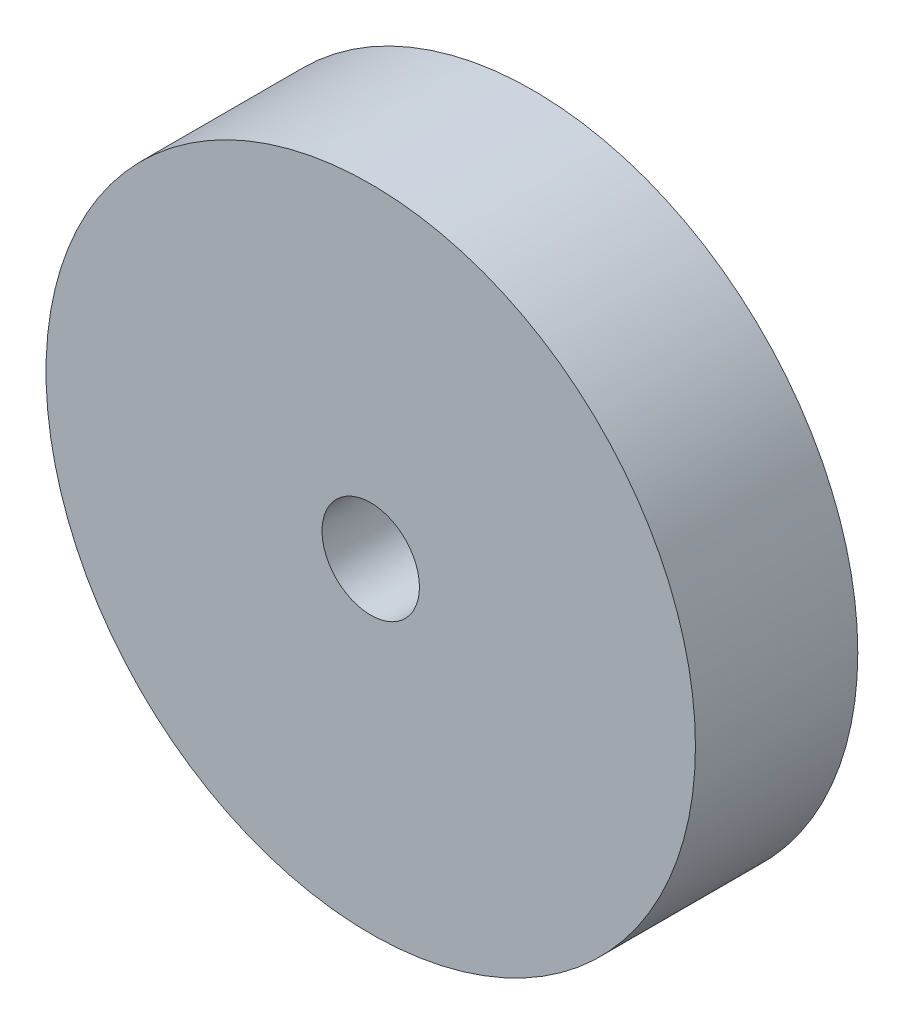
SolidWorks part; units mm, degrees
material "柔性聚氨酯泡沫体"
ref_plane "前视基准面" through (0, 0, 0) normal (0, 0, 1) x (1, 0, 0)
ref_plane "上视基准面" through (0, 0, 0) normal (0, 1, 0) x (1, 0, 0)
ref_plane "右视基准面" through (0, 0, 0) normal (1, 0, 0) x (0, 0, -1)
other "Configuration Table"
sketch "草图1" plane through (0, 0, 0) normal (0, 1, 0) x (1, 0, 0)
  line L0 (0, -129.0631) -> (0, 6324.094) construction
  line L1 (-3, 0) -> (-20, 0)
  line L2 (-20, 0) -> (-20, 10)
  line L3 (-20, 10) -> (-3, 10)
  line L4 (-3, 10) -> (-3, 0)
  dimension "D1" = 6
  dimension "D2" = 40
  dimension "D3" = 10
revolve "旋转1" add sketch "草图1" angle 360 about L0
